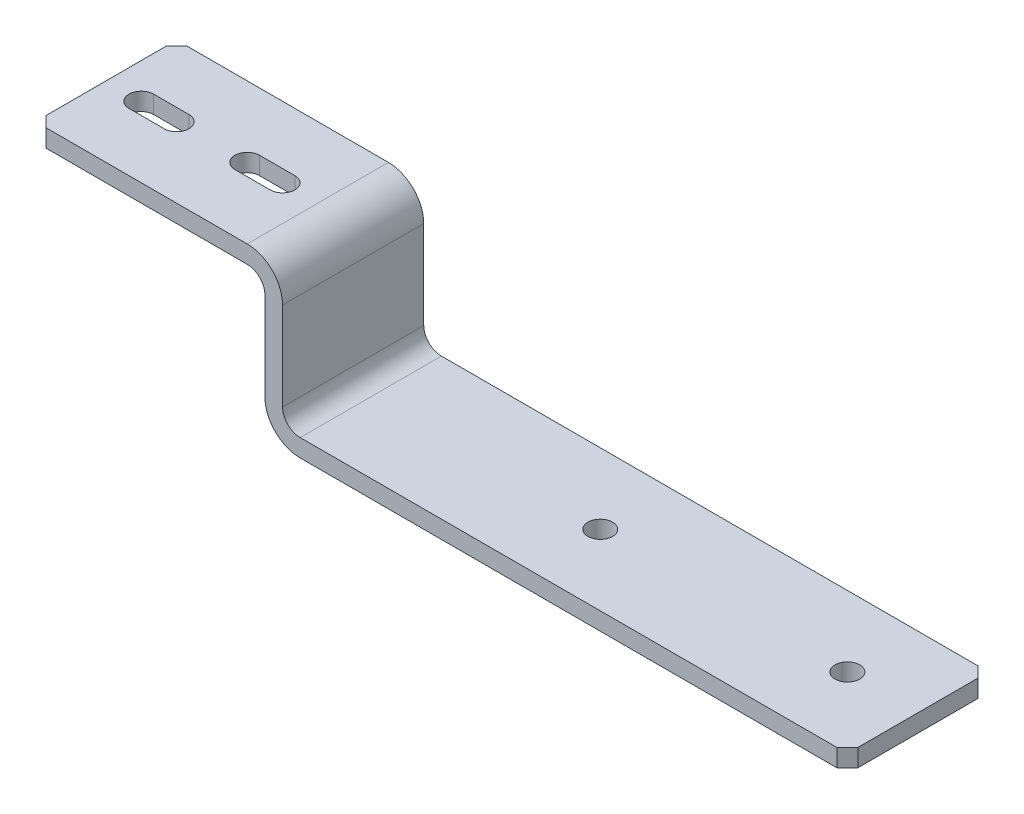
SolidWorks part; units mm, degrees
material "1023 碳钢板 (SS)"
ref_plane "Front Plane" through (0, 0, 0) normal (0, 0, 1) x (1, 0, 0)
ref_plane "Top Plane" through (0, 0, 0) normal (0, 1, 0) x (1, 0, 0)
ref_plane "Right Plane" through (0, 0, 0) normal (1, 0, 0) x (0, 0, -1)
sketch "Sketch1" plane through (0, 0, 0) normal (0, 0, 1) x (1, 0, 0)
  line L0 (0, 0) -> (60, 0)
  line L1 (65, -5) -> (65, -30)
  line L2 (75, -40) -> (230, -40)
  line L3 (0, 5) -> (60, 5)
  line L4 (70, -5) -> (70, -30)
  line L5 (75, -35) -> (230, -35)
  line L6 (0, 5) -> (0, 0)
  line L7 (230, -35) -> (230, -40)
  arc A0 (65, -30) -> (75, -40) centre (75, -30) ccw
  arc A1 (60, 0) -> (65, -5) centre (60, -5) cw
  arc A2 (60, 5) -> (70, -5) centre (60, -5) cw
  arc A3 (70, -30) -> (75, -35) centre (75, -30) ccw
  point P7 (65, -40)
  point P10 (65, 0)
  dimension "D4" = 10
  dimension "D5" = 5
  dimension "D1" = 65
  dimension "D2" = 165
  dimension "D3" = 40
  dimension "D6" = 5
extrude "Boss-Extrude1" add sketch "Sketch1" along normal blind 40 contours L7 L2 A0 L1 A1 L0 L6 L3 A2 L4 A3 L5
sketch "Sketch2" plane through (0, 5, 0) normal (0, 1, 0) x (1, 0, 0)
  line L0 (10, -20) -> (20, -20) construction
  line L1 (10, -16.5) -> (20, -16.5)
  line L2 (10, -23.5) -> (20, -23.5)
  line L3 (40, -20) -> (50, -20) construction
  line L4 (40, -16.5) -> (50, -16.5)
  line L5 (40, -23.5) -> (50, -23.5)
  line L6 (0, -40) -> (0, 0) construction
  arc A0 (10, -16.5) -> (10, -23.5) centre (10, -20) ccw
  arc A1 (20, -23.5) -> (20, -16.5) centre (20, -20) ccw
  arc A2 (40, -16.5) -> (40, -23.5) centre (40, -20) ccw
  arc A3 (50, -23.5) -> (50, -16.5) centre (50, -20) ccw
  point P2 (15, -20)
  point P7 (45, -20)
  point P17 (0, -20)
  dimension "D2" = 3.5
  dimension "D4" = 20
  dimension "D1" = 10
  dimension "D3" = 10
extrude "Cut-Extrude1" cut sketch "Sketch2" against normal blind 40
sketch "Sketch3" plane through (0, -35, 0) normal (0, 1, 0) x (1, 0, 0)
  line L0 (230, -40) -> (230, 0) construction
  circle A0 centre (140, -20) radius 3.5
  circle A1 centre (210, -20) radius 3.5
  point P7 (230, -20)
  dimension "D1" = 7
  dimension "D2" = 20
  dimension "D3" = 70
extrude "Cut-Extrude2" cut sketch "Sketch3" against normal blind 40
chamfer "Chamfer1" distance 3 angle 45 4 edges at (0, 2.5, 40) (0, 2.5, 0) (230, -37.5, 40) (230, -37.5, 0)
